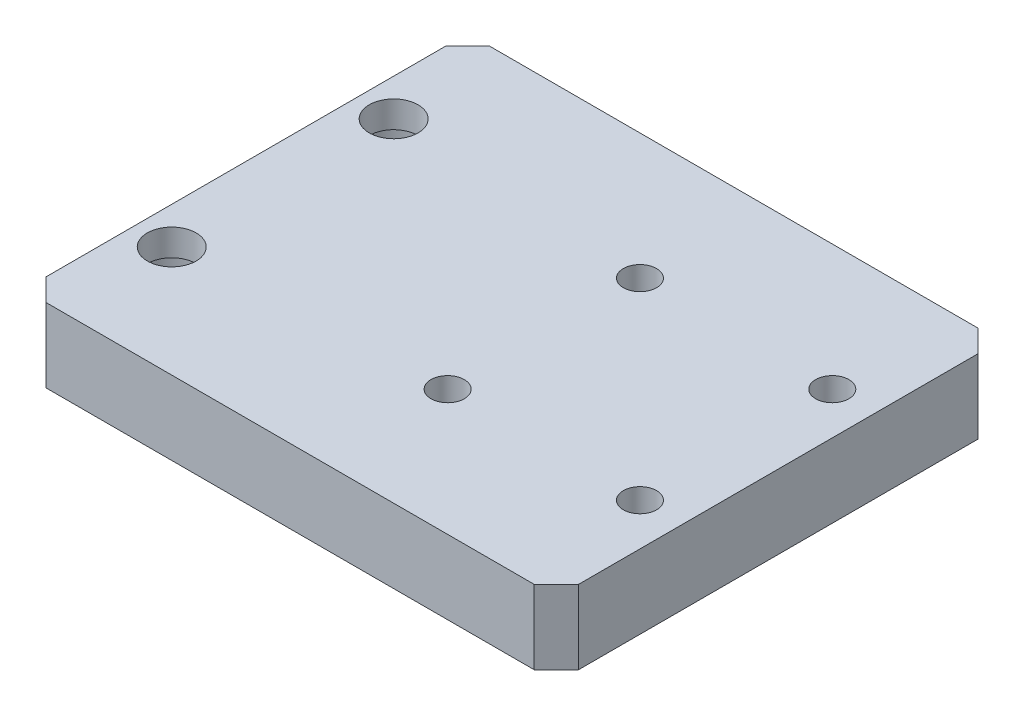
from build123d import *

# Parameters (mm, degrees)
EXTRUDE_1_DEPTH                = 60
HOLE_WIZARD_M6_2_D             = 5
HOLE_WIZARD_M6_2_DEPTH         = 17
HOLE_WIZARD_M6_2_TIP           = 1.502151548
HOLE_WIZARD_M4_1_D             = 4.5
HOLE_WIZARD_M4_1_DEPTH         = 11.5
HOLE_WIZARD_M4_1_CBORE_D       = 8
HOLE_WIZARD_M4_1_CBORE_DEPTH   = 4.4
HOLE_WIZARD_M4_1_TIP           = 1.351936393
HOLE_WIZARD_M6_1_D             = 5
HOLE_WIZARD_M6_1_DEPTH         = 17
HOLE_WIZARD_M6_1_TIP           = 1.502151548
CHAMFER_1_SIZE                 = 3
SKETCH_9_W                     = 10
SKETCH_9_H                     = 44
CUT_EXTRUDE_1_DEPTH            = 109.166538369
CHAMFER_2_SIZE                 = 3
HOLE_WIZARD_M6_1_2_D           = 6.6
HOLE_WIZARD_M6_1_2_DEPTH       = 17
HOLE_WIZARD_M6_1_2_CBORE_D     = 11
HOLE_WIZARD_M6_1_2_CBORE_DEPTH = 6.4
HOLE_WIZARD_M6_1_2_TIP         = 1.982840043


with BuildPart() as part:
    # 草图2 → 凸台-拉伸1 (new body)
    with BuildSketch(Plane.XY):
        Polygon((0, 0), (0, -54), (72, -54), (72, -44), (10, -44), (10, 0), align=None)
    extrude(amount=EXTRUDE_1_DEPTH)

    # M6 螺纹孔2
    with Locations(Plane(origin=(0, 0, 0), x_dir=(-1, 0, 0), z_dir=(0, 0, -1))):
        with Locations((-60, -49)):
            Hole(HOLE_WIZARD_M6_2_D / 2, depth=HOLE_WIZARD_M6_2_DEPTH)
            with Locations((0, 0, -(HOLE_WIZARD_M6_2_DEPTH + HOLE_WIZARD_M6_2_TIP / 2))):  # 118° drill point
                Cone(0, HOLE_WIZARD_M6_2_D / 2, HOLE_WIZARD_M6_2_TIP, mode=Mode.SUBTRACT)

    # M4 六角凹头螺钉的柱形沉头孔1
    with Locations(Plane(origin=(0, -54, 0), x_dir=(-1, 0, 0), z_dir=(0, -1, 0))):
        with Locations((-40.299995099, -17), (-66.299995099, -17), (-66.299995099, -43), (-40.299995099, -43)):
            CounterBoreHole(HOLE_WIZARD_M4_1_D / 2, HOLE_WIZARD_M4_1_CBORE_D / 2, HOLE_WIZARD_M4_1_CBORE_DEPTH, depth=HOLE_WIZARD_M4_1_DEPTH)
            with Locations((0, 0, -(HOLE_WIZARD_M4_1_DEPTH + HOLE_WIZARD_M4_1_TIP / 2))):  # 118° drill point
                Cone(0, HOLE_WIZARD_M4_1_D / 2, HOLE_WIZARD_M4_1_TIP, mode=Mode.SUBTRACT)

    # Hole Wizard M6 _1
    with Locations(Plane(origin=(0, 0, 0), x_dir=(1, 0, 0), z_dir=(0, 1, 0))):
        with Locations((5, -15), (5, -45)):
            Hole(HOLE_WIZARD_M6_1_D / 2, depth=HOLE_WIZARD_M6_1_DEPTH)
            with Locations((0, 0, -(HOLE_WIZARD_M6_1_DEPTH + HOLE_WIZARD_M6_1_TIP / 2))):  # 118° drill point
                Cone(0, HOLE_WIZARD_M6_1_D / 2, HOLE_WIZARD_M6_1_TIP, mode=Mode.SUBTRACT)

    # 倒角1
    chamfer_1_edges = [part.edges().sort_by_distance(p)[0] for p in [
        (72, -49, 60),
        (5, 0, 60),
        (72, -49, 0),
        (5, 0, 0),
    ]]
    chamfer(chamfer_1_edges, length=CHAMFER_1_SIZE)

    # 草图9 → 切除-拉伸1 (cut, through all)
    with BuildSketch(Plane.XY.offset(60)):
        with Locations((5, -22)):
            Rectangle(SKETCH_9_W, SKETCH_9_H)
    extrude(amount=-CUT_EXTRUDE_1_DEPTH, mode=Mode.SUBTRACT)

    # 倒角2
    chamfer_2_edges = [part.edges().sort_by_distance(p)[0] for p in [
        (0, -49, 0),
        (0, -49, 60),
    ]]
    chamfer(chamfer_2_edges, length=CHAMFER_2_SIZE)

    # Hole Wizard M6 _1 2
    with Locations(Plane(origin=(0, -54, 0), x_dir=(-1, 0, 0), z_dir=(0, -1, 0))):
        with Locations((-5, -15), (-5, -45)):
            CounterBoreHole(HOLE_WIZARD_M6_1_2_D / 2, HOLE_WIZARD_M6_1_2_CBORE_D / 2, HOLE_WIZARD_M6_1_2_CBORE_DEPTH, depth=HOLE_WIZARD_M6_1_2_DEPTH)
            with Locations((0, 0, -(HOLE_WIZARD_M6_1_2_DEPTH + HOLE_WIZARD_M6_1_2_TIP / 2))):  # 118° drill point
                Cone(0, HOLE_WIZARD_M6_1_2_D / 2, HOLE_WIZARD_M6_1_2_TIP, mode=Mode.SUBTRACT)


solid = part.part
